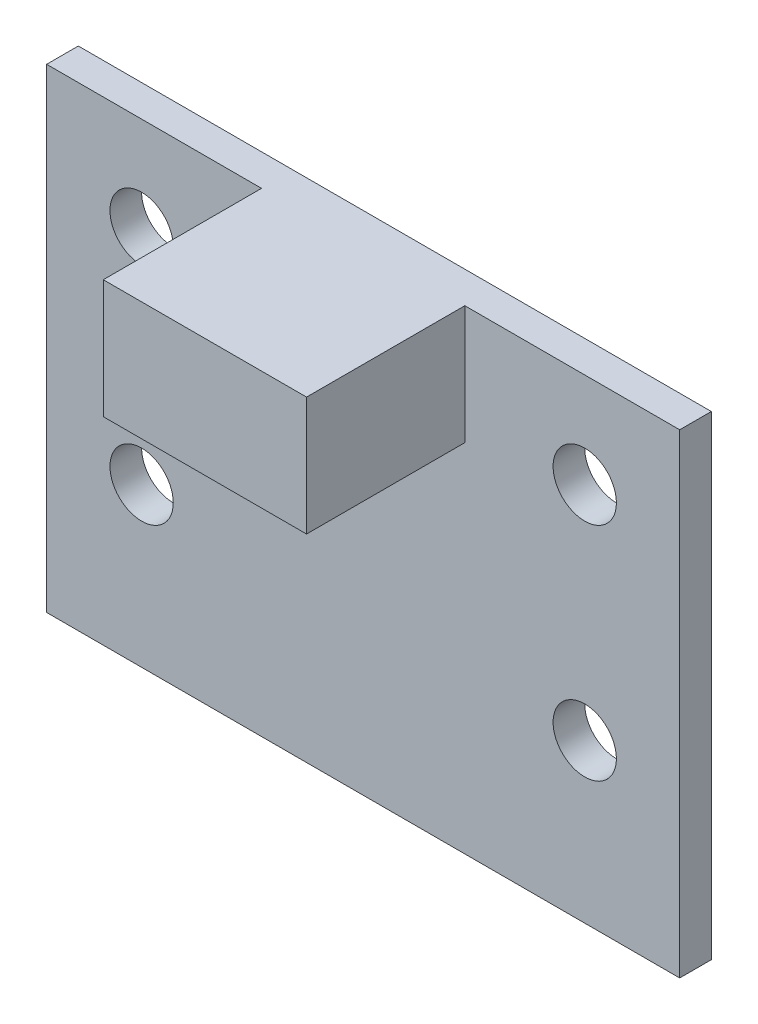
SolidWorks part; units mm, degrees
ref_plane "Front Plane" through (0, 0, 0) normal (0, 0, 1) x (1, 0, 0)
ref_plane "Top Plane" through (0, 0, 0) normal (0, 1, 0) x (1, 0, 0)
ref_plane "Right Plane" through (0, 0, 0) normal (1, 0, 0) x (0, 0, -1)
other "Configuration Table"
sketch "Sketch1" plane through (0, 0, 0) normal (0, 0, 1) x (1, 0, 0)
  line L1 (-10, 7.5) -> (10, 7.5)
  line L2 (-10, 7.5) -> (-10, -7.5)
  line L3 (-10, -7.5) -> (10, -7.5)
  line L4 (10, 7.5) -> (10, -7.5)
  line L5 (-10, 7.5) -> (10, -7.5) construction
  line L6 (-10, -7.5) -> (10, 7.5) construction
  line L7 (-7, 4.5) -> (7, 4.5) construction
  line L8 (-7, 4.5) -> (-7, -2.5) construction
  line L9 (-7, -2.5) -> (7, -2.5) construction
  line L10 (7, 4.5) -> (7, -2.5) construction
  circle A4 centre (-7, 4.5) radius 1
  circle A5 centre (-7, -2.5) radius 1
  circle A6 centre (7, 4.5) radius 1
  circle A7 centre (7, -2.5) radius 1
  point P0 (0, 0)
  point P6 (0, 0)
  dimension "D5" = 3
  dimension "D6" = 2
  dimension "D7" = 3
  dimension "D1" = 20
  dimension "D2" = 15
  dimension "D3" = 3
  dimension "D4" = 5
extrude "Boss-Extrude1" add sketch "Sketch1" along normal blind 1
sketch "Sketch2" plane through (0, 0, 1) normal (0, 0, 1) x (1, 0, 0)
  line L1 (-3.211, 7.5) -> (3.211, 7.5)
  line L2 (-3.211, 7.5) -> (-3.211, 3.7526)
  line L3 (-3.211, 3.7526) -> (3.211, 3.7526)
  line L4 (3.211, 7.5) -> (3.211, 3.7526)
  line L5 (-3.211, 7.5) -> (3.211, 3.7526) construction
  line L6 (-3.211, 3.7526) -> (3.211, 7.5) construction
  line L7 (10, 7.5) -> (-10, 7.5) construction
  point P0 (0, 5.6263)
extrude "Boss-Extrude2" add sketch "Sketch2" along normal blind 5
